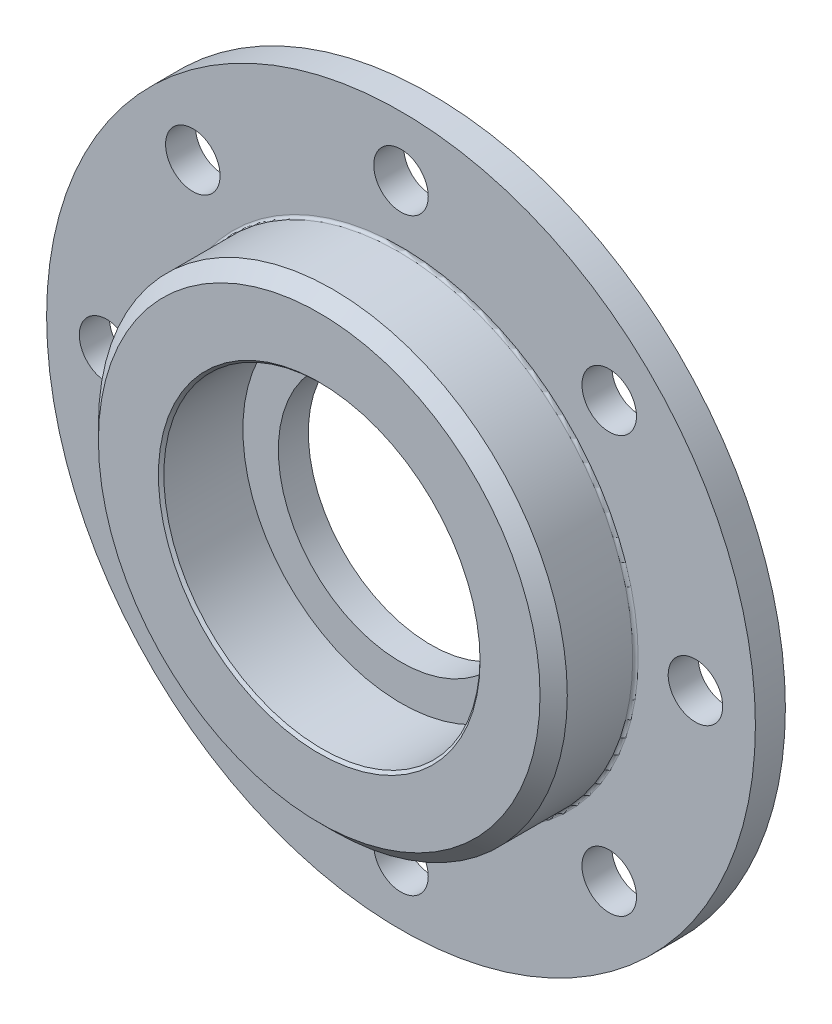
SolidWorks part; units mm, degrees
material "灰铸铁"
ref_plane "前视基准面" through (0, 0, 0) normal (0, 0, 1) x (1, 0, 0)
ref_plane "上视基准面" through (0, 0, 0) normal (0, 1, 0) x (1, 0, 0)
ref_plane "右视基准面" through (0, 0, 0) normal (1, 0, 0) x (0, 0, -1)
sketch "草图1" plane through (0, 0, 0) normal (0, 0, 1) x (1, 0, 0)
  circle A0 centre (0, 0) radius 130
extrude "凸台-拉伸1" add sketch "草图1" along normal blind 11
sketch "草图2" plane through (0, 0, 11) normal (0, 0, 1) x (1, 0, 0)
  circle A0 centre (0, 0) radius 58
  circle A1 centre (0, 0) radius 86
  dimension "D1" = 28
extrude "凸台-拉伸2" add sketch "草图2" along normal blind 30 contours A0 | A1
fillet "圆角1" radius 1 1 edges at (86, 0, 11)
chamfer "倒角1" distance 1 angle 45 1 edges at (58, 0, 41)
chamfer "倒角2" distance 5 angle 45 1 edges at (86, 0, 41)
sketch "草图4" plane through (0, 0, 0) normal (0, 0, -1) x (-1, 0, 0)
  circle A0 centre (0, 0) radius 108 construction
  circle A1 centre (0, 108) radius 10
extrude "切除-拉伸1" cut sketch "草图4" against normal up to next
pattern_circular "阵列(圆周)1" count 8 over 360 about axis through (0, 0, 0) along (0, 0, 1) of "切除-拉伸1"
sketch "草图5" plane through (0, 0, 11) normal (0, 0, 1) x (1, 0, 0)
  circle A0 centre (0, 0) radius 40 construction
  circle A1 centre (0, 0) radius 51.5 construction
  circle A2 centre (0, 0) radius 45
extrude "切除-拉伸2" cut sketch "草图5" against normal through all
